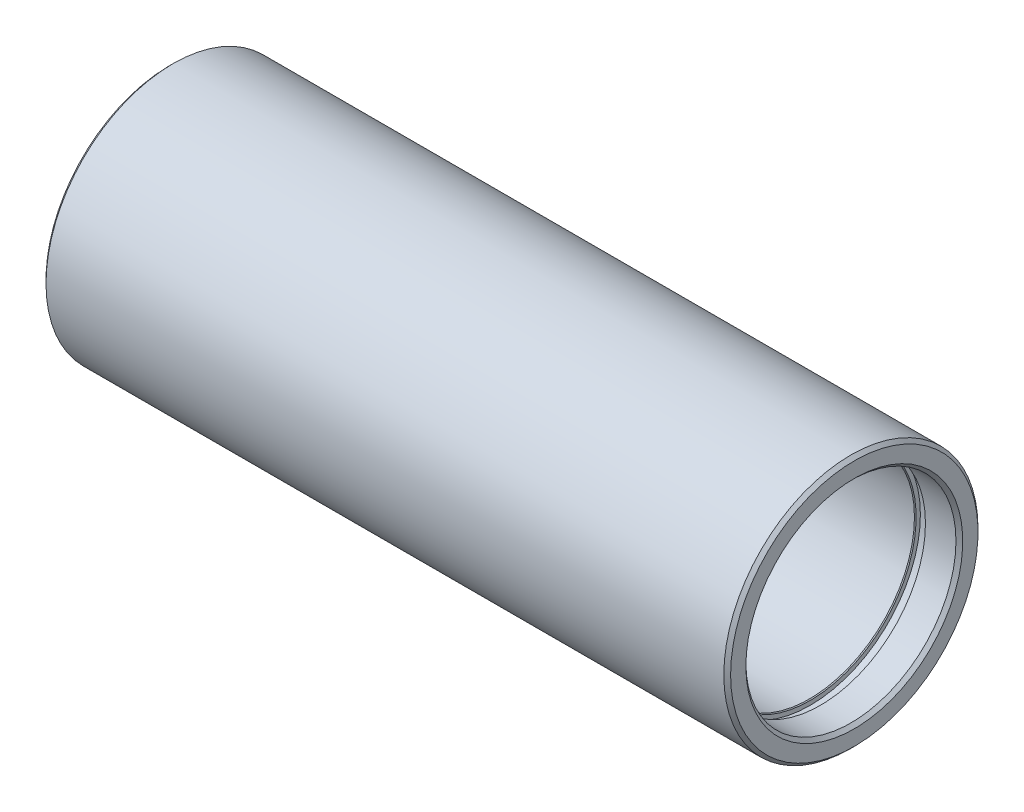
from build123d import *

# Parameters (mm, degrees)
CHAMFER_1_SIZE = 1
CHAMFER_2_SIZE = 0.25


with BuildPart() as part:
    # 草图1 → 旋转1 (revolve)
    with BuildSketch(Plane.XY, mode=Mode.PRIVATE) as revolve_1_sk:
        Polygon((-4.124391585, 31), (5.875608415, 31), (5.875608415, 32.5), (8.875608415, 32.5), (8.875608415, 31), (184.875608415, 31), (184.875608415, 32.5), (187.875608415, 32.5), (187.875608415, 31), (197.875608415, 31), (197.875608415, 37.5), (-4.124391585, 37.5), align=None)
    revolve(revolve_1_sk.sketch.rotate(Axis((0, 0, 0), (1, 0, 0)), 90), axis=Axis((0, 0, 0), (1, 0, 0)))

    # 倒角1
    chamfer_1_edges = [part.edges().sort_by_distance(p)[0] for p in [
        (197.875608415, 0, -31),
        (197.875608415, 0, -37.5),
        (-4.124391585, 0, -37.5),
        (-4.124391585, 0, -31),
    ]]
    chamfer(chamfer_1_edges, length=CHAMFER_1_SIZE)

    # 倒角2
    chamfer_2_edges = [part.edges().sort_by_distance(p)[0] for p in [
        (8.875608415, 0, -31),
        (184.875608415, 0, -31),
    ]]
    chamfer(chamfer_2_edges, length=CHAMFER_2_SIZE)


solid = part.part
